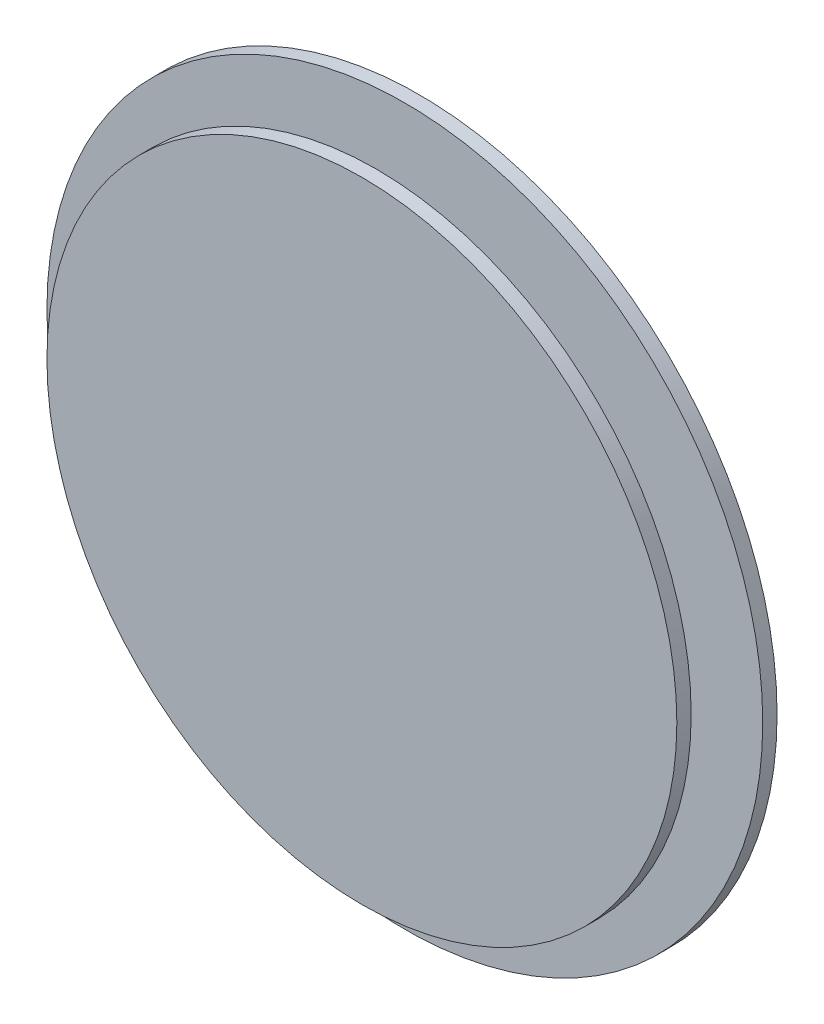
from build123d import *

# Parameters (mm, degrees)
SKETCH_3_R           = 25
BOSS_EXTRUDE_1_DEPTH = 1
SKETCH_4_R           = 19
BOSS_EXTRUDE_2_DEPTH = 2
SKETCH_5_R           = 22
BOSS_EXTRUDE_3_DEPTH = 1


with BuildPart() as part:
    # Sketch 3 → Boss-Extrude 1 (new body)
    with BuildSketch(Plane.XY):
        Circle(SKETCH_3_R)
    extrude(amount=BOSS_EXTRUDE_1_DEPTH)

    # Sketch 4 → Boss-Extrude 2 (add)
    with BuildSketch(Plane.XY.offset(1)):
        Circle(SKETCH_4_R)
    extrude(amount=BOSS_EXTRUDE_2_DEPTH)

    # Sketch 5 → Boss-Extrude 3 (add)
    with BuildSketch(Plane.XY.offset(3)):
        Circle(SKETCH_5_R)
    extrude(amount=BOSS_EXTRUDE_3_DEPTH)


solid = part.part
